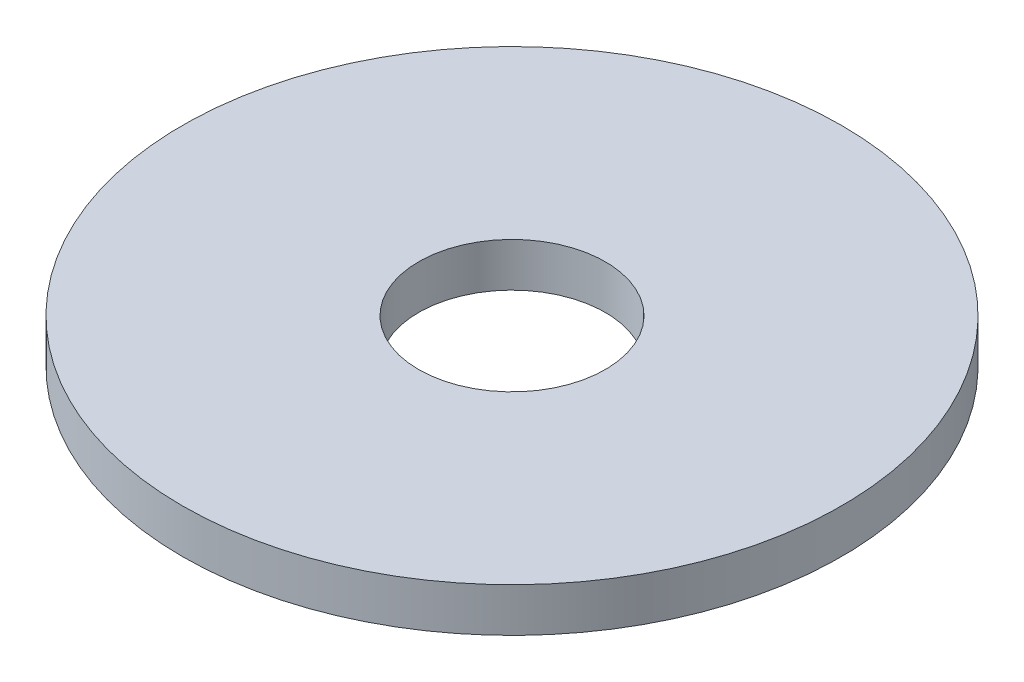
SolidWorks part; units mm, degrees
material "Q235B"
ref_plane "Front" through (0, 0, 0) normal (0, 0, 1) x (1, 0, 0)
ref_plane "Top" through (0, 0, 0) normal (0, 1, 0) x (1, 0, 0)
ref_plane "Right" through (0, 0, 0) normal (1, 0, 0) x (0, 0, -1)
sketch "Sketch1" plane through (0, 0, 0) normal (0, 1, 0) x (1, 0, 0)
  circle A0 centre (0, 0) radius 8.5
  circle A1 centre (0, 0) radius 30
  dimension "D1" = 17
  dimension "D2" = 60
extrude "Extrude1" add sketch "Sketch1" along normal mid plane 4
